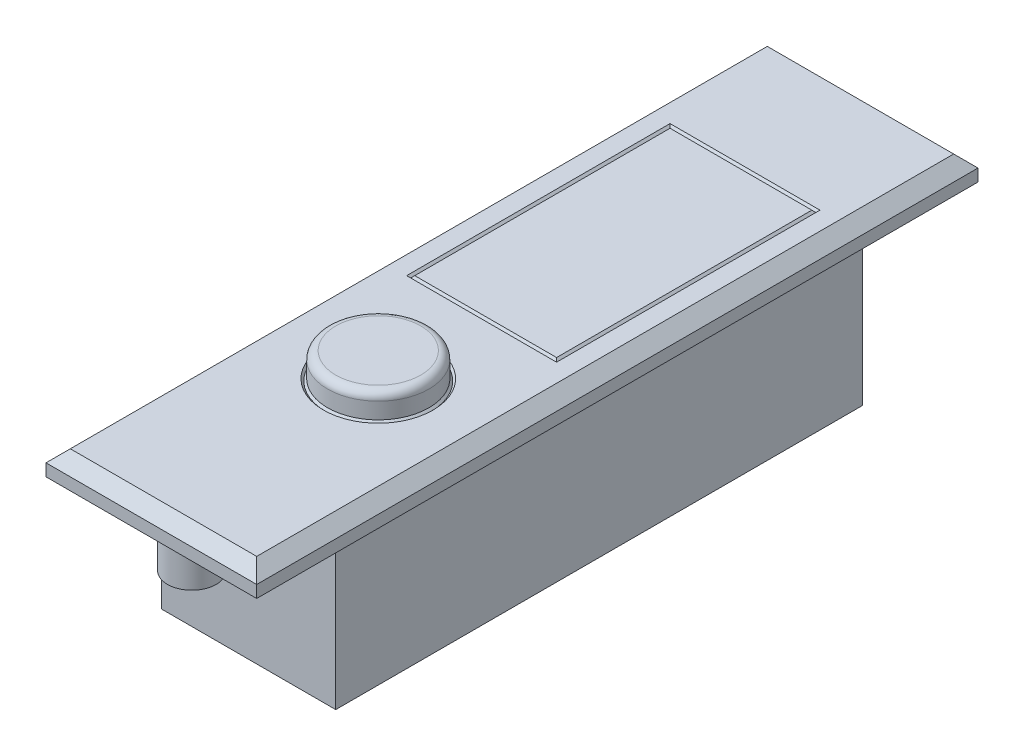
from build123d import *

# Parameters (mm, degrees)
SKETCH1_W               = 26
SKETCH1_H               = 89
BOSS_EXTRUDE1_DEPTH     = 3
SKETCH2_R               = 6.75
SKETCH2_R_2             = 6.25
SKETCH2_W               = 18.5
SKETCH2_H               = 32.5
SKETCH2_W_2             = 17.5
SKETCH2_H_2             = 31.5
CUT_EXTRUDE_THIN1_DEPTH = 1
CUT_EXTRUDE_THIN1_TAPER = 44
SKETCH3_R               = 6.25
BOSS_EXTRUDE2_DEPTH     = 3
FILLET1_R               = 1
CHAMFER1_SIZE           = 1.5
SKETCH4_R               = 3
SKETCH4_R_2             = 2
EXTRUDE_THIN2_DEPTH     = 6
SKETCH5_W               = 21.5
SKETCH5_H               = 65
BOSS_EXTRUDE3_DEPTH     = 19


with BuildPart() as part:
    # Sketch1 → Boss-Extrude1 (new body)
    with BuildSketch(Plane(origin=(0, 0, 0), x_dir=(1, 0, 0), z_dir=(0, 1, 0))):
        Rectangle(SKETCH1_W, SKETCH1_H)
    extrude(amount=BOSS_EXTRUDE1_DEPTH)

    # Sketch2 → Cut-Extrude-Thin1 (cut)
    # profile 1 of 2: a face of its own
    with BuildSketch(Plane(origin=(0, 3, 0), x_dir=(1, 0, 0), z_dir=(0, 1, 0))):
        with Locations((0, -16.5)):
            Circle(SKETCH2_R)
        with Locations((0, -16.5)):
            Circle(SKETCH2_R_2, mode=Mode.SUBTRACT)
    # profile 2 of 2: a face of its own
    with BuildSketch(Plane(origin=(0, 3, 0), x_dir=(1, 0, 0), z_dir=(0, 1, 0))):
        with Locations((0, 12.5)):
            Rectangle(SKETCH2_W, SKETCH2_H)
        with Locations((0, 12.5)):
            Rectangle(SKETCH2_W_2, SKETCH2_H_2, mode=Mode.SUBTRACT)
    extrude(amount=-CUT_EXTRUDE_THIN1_DEPTH, taper=CUT_EXTRUDE_THIN1_TAPER, mode=Mode.SUBTRACT)

    # Sketch3 → Boss-Extrude2 (add)
    with BuildSketch(Plane(origin=(0, 3, 0), x_dir=(1, 0, 0), z_dir=(0, 1, 0))):
        with Locations((0, -16.5)):
            Circle(SKETCH3_R)
    extrude(amount=BOSS_EXTRUDE2_DEPTH)

    # Fillet1
    fillet1_edges = [part.edges().sort_by_distance(p)[0] for p in [
        (-6.25, 6, 16.5),
    ]]
    fillet(fillet1_edges, radius=FILLET1_R)

    # Chamfer1
    chamfer1_edges = [part.edges().sort_by_distance(p)[0] for p in [
        (-13, 3, 0),
        (0, 3, 44.5),
        (13, 3, 0),
        (0, 3, -44.5),
    ]]
    chamfer(chamfer1_edges, length=CHAMFER1_SIZE)

    # Sketch4 → Extrude-Thin2 (add)
    # profile 1 of 2: a face of its own
    with BuildSketch(Plane.XZ):
        with Locations((0, -39.5)):
            Circle(SKETCH4_R)
        with Locations((0, -39.5)):
            Circle(SKETCH4_R_2, mode=Mode.SUBTRACT)
    # profile 2 of 2: a face of its own
    with BuildSketch(Plane.XZ):
        with Locations((0, 39.5)):
            Circle(SKETCH4_R)
        with Locations((0, 39.5)):
            Circle(SKETCH4_R_2, mode=Mode.SUBTRACT)
    extrude(amount=EXTRUDE_THIN2_DEPTH)

    # Sketch5 → Boss-Extrude3 (add)
    with BuildSketch(Plane.XZ):
        Rectangle(SKETCH5_W, SKETCH5_H)
    extrude(amount=BOSS_EXTRUDE3_DEPTH)


solid = part.part
